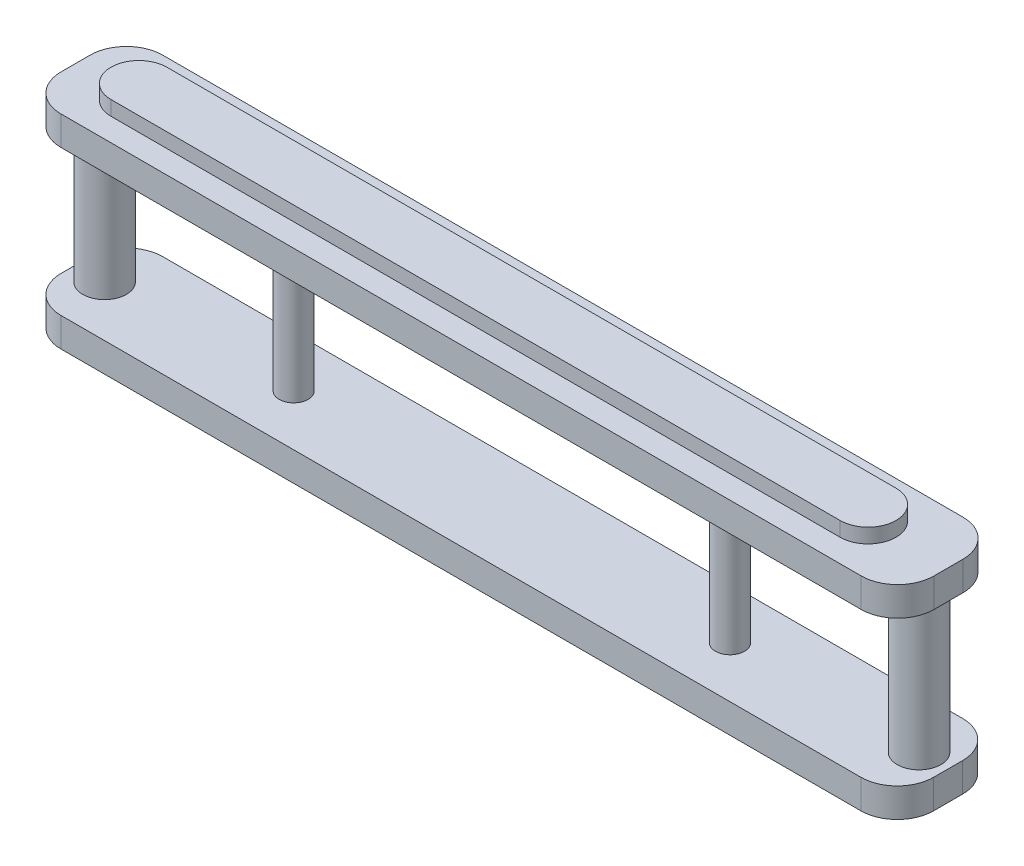
from build123d import *

# Parameters (mm, degrees)
SKETCH3_W           = 6000
SKETCH3_H           = 700
BOSS_EXTRUDE3_DEPTH = 200
SKETCH4_R           = 150
SKETCH4_R_2         = 100
BOSS_EXTRUDE4_DEPTH = 1000
SKETCH5_W           = 6002.219419971
SKETCH5_H           = 700
BOSS_EXTRUDE5_DEPTH = 200
FILLET1_R           = 250
BOSS_EXTRUDE6_DEPTH = 100


with BuildPart() as part:
    # Sketch3 → Boss-Extrude3 (new body)
    with BuildSketch(Plane(origin=(0, 0, 0), x_dir=(1, 0, 0), z_dir=(0, 1, 0))):
        Rectangle(SKETCH3_W, SKETCH3_H)
    extrude(amount=BOSS_EXTRUDE3_DEPTH)

    # Sketch4 → Boss-Extrude4 (add)
    with BuildSketch(Plane(origin=(0, 200, 0), x_dir=(1, 0, 0), z_dir=(0, 1, 0))):
        with Locations(Location((-2800, 0, 0), (0, 0, 270))):
            Circle(SKETCH4_R)
        with Locations(Location((2800, 0, 0), (0, 0, 270))):
            Circle(SKETCH4_R)
        with Locations(Location((-1500, 0, 0), (0, 0, 270))):
            Circle(SKETCH4_R_2)
        with Locations(Location((1500, 0, 0), (0, 0, 270))):
            Circle(SKETCH4_R_2)
    extrude(amount=BOSS_EXTRUDE4_DEPTH)

    # Sketch5 → Boss-Extrude5 (add)
    with BuildSketch(Plane(origin=(0, 1200, 0), x_dir=(1, 0, 0), z_dir=(0, 1, 0))):
        with Locations((1.109709986, 0)):
            Rectangle(SKETCH5_W, SKETCH5_H)
    extrude(amount=BOSS_EXTRUDE5_DEPTH)

    # Fillet1
    fillet1_edges = [part.edges().sort_by_distance(p)[0] for p in [
        (3002.219419971, 1300, -350),
        (-3000, 1300, -350),
        (-3000, 1300, 350),
        (3002.219419971, 1300, 350),
        (3000, 100, 350),
        (-3000, 100, 350),
        (-3000, 100, -350),
        (3000, 100, -350),
    ]]
    fillet(fillet1_edges, radius=FILLET1_R)

    # Sketch6 → Boss-Extrude6 (add)
    with BuildSketch(Plane.XZ):
        with BuildLine():
            Line((-2564.072960881, 192.302850828), (2449.537078564, 192.302850828))
            ThreePointArc((2449.537078564, 192.302850828), (2641.839929392, 0), (2449.537078564, -192.302850828))
            Line((2449.537078564, -192.302850828), (-2564.072960881, -192.302850828))
            ThreePointArc((-2564.072960881, -192.302850828), (-2756.375811709, 0), (-2564.072960881, 192.302850828))
        make_face()
    boss_extrude6 = extrude(amount=BOSS_EXTRUDE6_DEPTH)

    # Mirror1: Boss-Extrude6 across plane
    add(boss_extrude6.mirror(Plane.ZX.offset(700)))


solid = part.part
